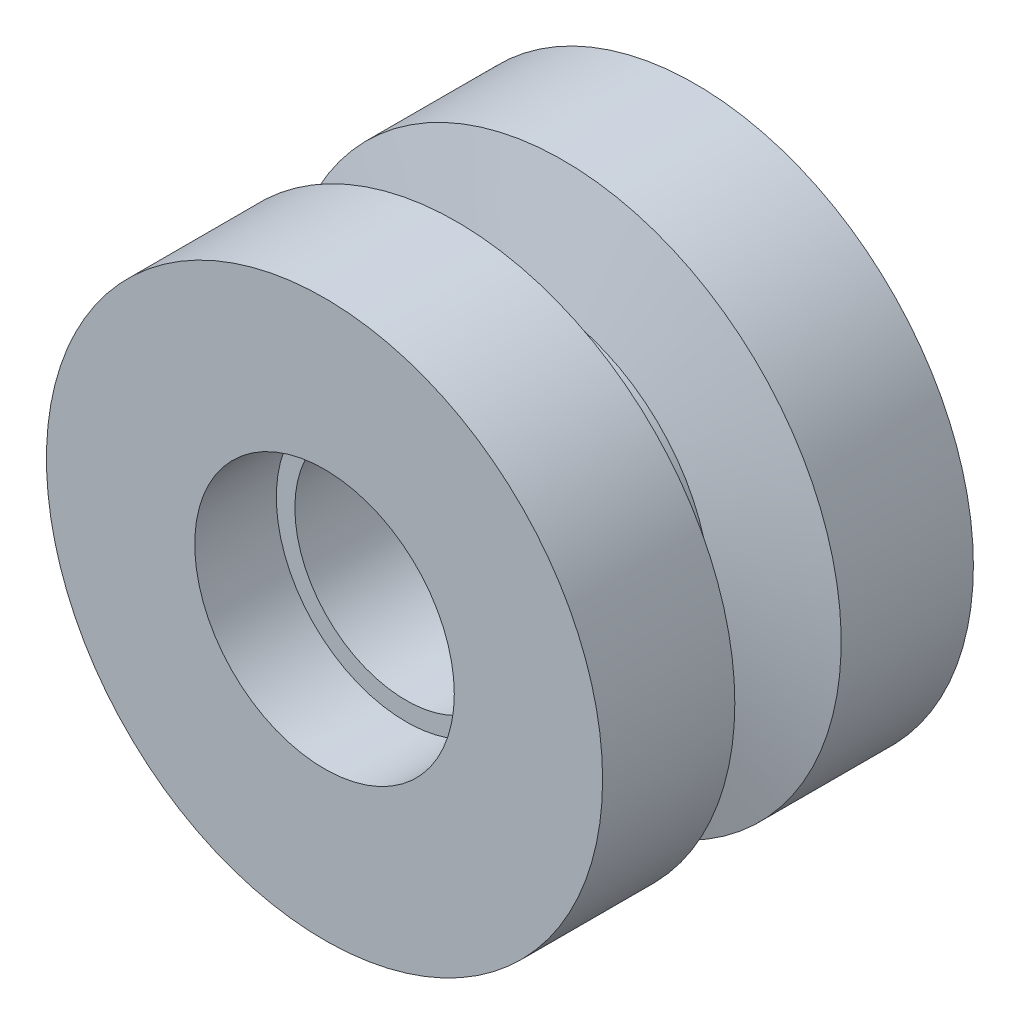
from build123d import *

# Parameters (mm, degrees)
SKETCH_1_R          = 37.5
SKETCH_1_R_2        = 15
EXTRUDE_1_DEPTH     = 50
SKETCH_3_R          = 17.5
CUT_EXTRUDE_1_DEPTH = 11
CUT_EXTRUDE_START   = -11
SKETCH_4_R          = 17.5
CUT_EXTRUDE_2_DEPTH = 11


with BuildPart() as part:
    # 草图1 → 凸台-拉伸1 (new body)
    with BuildSketch(Plane.XY):
        Circle(SKETCH_1_R)
        Circle(SKETCH_1_R_2, mode=Mode.SUBTRACT)
    extrude(amount=EXTRUDE_1_DEPTH)

    # 草图2 → 切除-旋转1 (revolve, cut)
    with BuildSketch(Plane(origin=(0, 0, 0), x_dir=(1, 0, 0), z_dir=(0, 1, 0))):
        Polygon((-38.25, -17.648818614), (-23.25, -21.25), (-23.25, -28.75), (-38.25, -32.351181386), align=None)
    revolve(axis=Axis((0, 0, 0), (0, 0, 1)), mode=Mode.SUBTRACT)

    # 草图3 → 切除-拉伸1 (cut)
    with BuildSketch(Plane.XY.offset(50)):
        Circle(SKETCH_3_R)
    extrude(amount=-CUT_EXTRUDE_1_DEPTH, mode=Mode.SUBTRACT)

    # 草图4 → 切除-拉伸2 (cut)
    with BuildSketch(Plane(origin=(0, 0, 0), x_dir=(-1, 0, 0), z_dir=(0, 0, -1)).offset(CUT_EXTRUDE_START)):
        with Locations(Location((0, 0, 0), (0, 0, 180))):
            Circle(SKETCH_4_R)
    extrude(amount=CUT_EXTRUDE_2_DEPTH, mode=Mode.SUBTRACT)


solid = part.part
